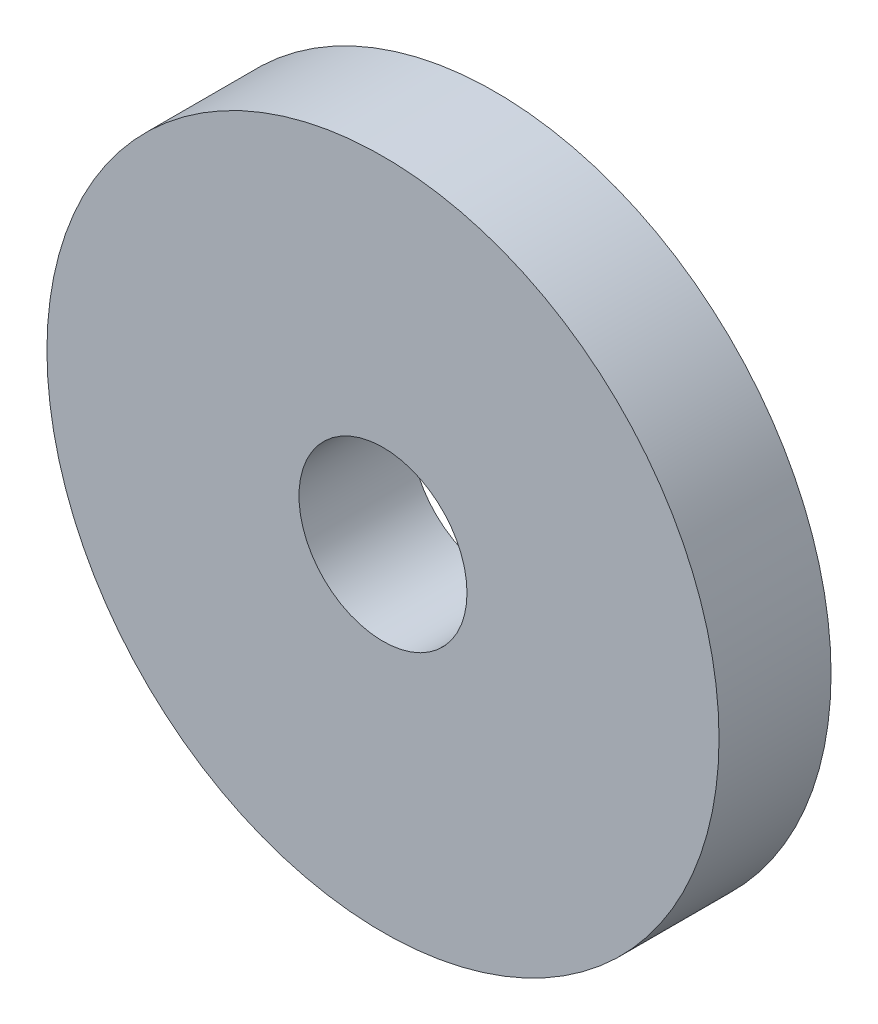
SolidWorks part; units mm, degrees
ref_plane "前视基准面" through (0, 0, 0) normal (0, 0, 1) x (1, 0, 0)
ref_plane "上视基准面" through (0, 0, 0) normal (0, 1, 0) x (1, 0, 0)
ref_plane "右视基准面" through (0, 0, 0) normal (1, 0, 0) x (0, 0, -1)
sketch "草图1" plane through (0, 0, 0) normal (0, 0, 1) x (1, 0, 0)
  circle A0 centre (0, 0) radius 15
  circle A1 centre (0, 0) radius 60
  point P5 (0, -0.1213)
  dimension "D1" = 30
  dimension "D2" = 120
extrude "凸台-拉伸1" add sketch "草图1" along normal mid plane 20
